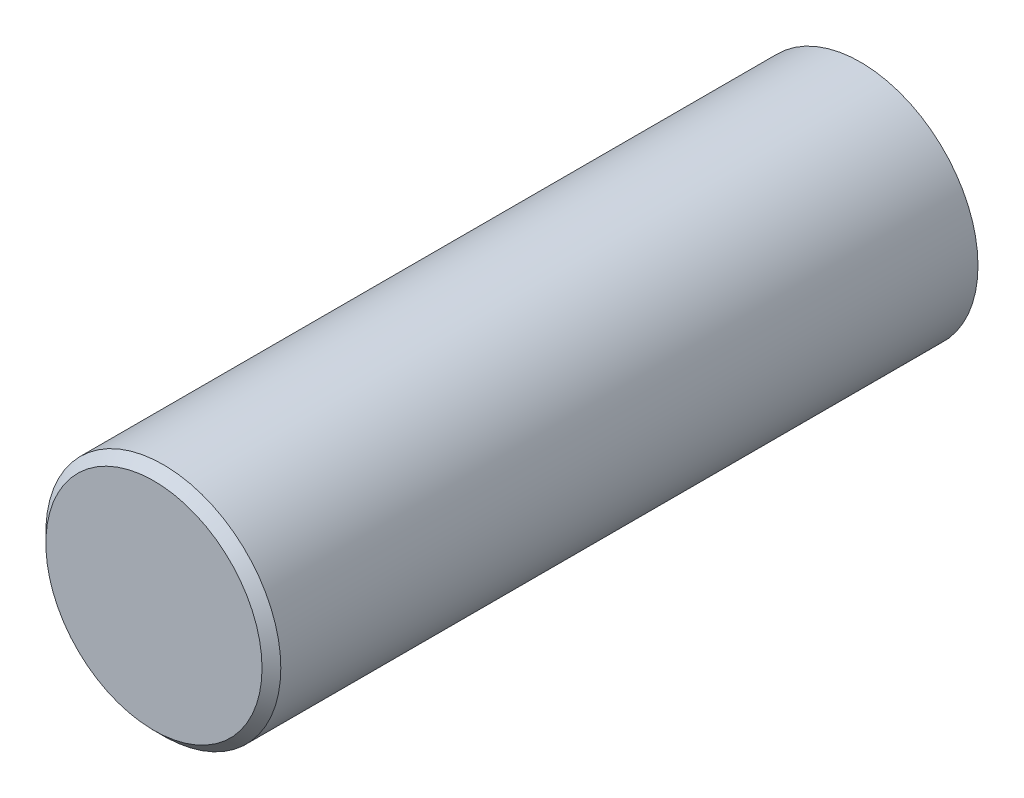
from build123d import *

# Parameters (mm, degrees)
SKETCH1_R           = 62.5
BOSS_EXTRUDE1_DEPTH = 345.880548662
BOSS_EXTRUDE2_START = 10
BOSS_EXTRUDE2_DEPTH = 10
BOSS_EXTRUDE3_START = 20
SKETCH4_R           = 62.5
BOSS_EXTRUDE3_DEPTH = 20
CHAMFER1_SIZE       = 5


with BuildPart() as part:
    # Sketch1 → Boss-Extrude1 (new body)
    with BuildSketch(Plane.XY):
        with Locations((5089.410855653, 2238.406272837)):
            Circle(SKETCH1_R)
    extrude(amount=-BOSS_EXTRUDE1_DEPTH)

    # Sketch3 → Boss-Extrude2 (add)
    with BuildSketch(Plane.XY.offset(BOSS_EXTRUDE2_START)):
        with BuildLine():
            Line((5056.406144678, 2185.331428951), (5095.721720008, 2190.511896514))
            Line((5095.721720008, 2190.511896514), (5135.037295338, 2195.692364076))
            ThreePointArc((5135.037295338, 2195.692364076), (5147.539602759, 2215.443286101), (5151.910855653, 2238.406272837))
            ThreePointArc((5151.910855653, 2238.406272837), (5059.050885593, 2293.037053702), (5056.406144678, 2185.331428951))
        make_face()
    extrude(amount=-BOSS_EXTRUDE2_DEPTH)

    # Sketch4 → Boss-Extrude3 (add)
    with BuildSketch(Plane.XY.offset(10).offset(BOSS_EXTRUDE3_START)):
        with Locations((5089.410855653, 2238.406272837)):
            Circle(SKETCH4_R)
    extrude(amount=-BOSS_EXTRUDE3_DEPTH)

    # Chamfer1
    chamfer1_edges = [part.edges().sort_by_distance(p)[0] for p in [
        (5026.910855653, 2238.406272837, 30),
    ]]
    chamfer(chamfer1_edges, length=CHAMFER1_SIZE)


solid = part.part
